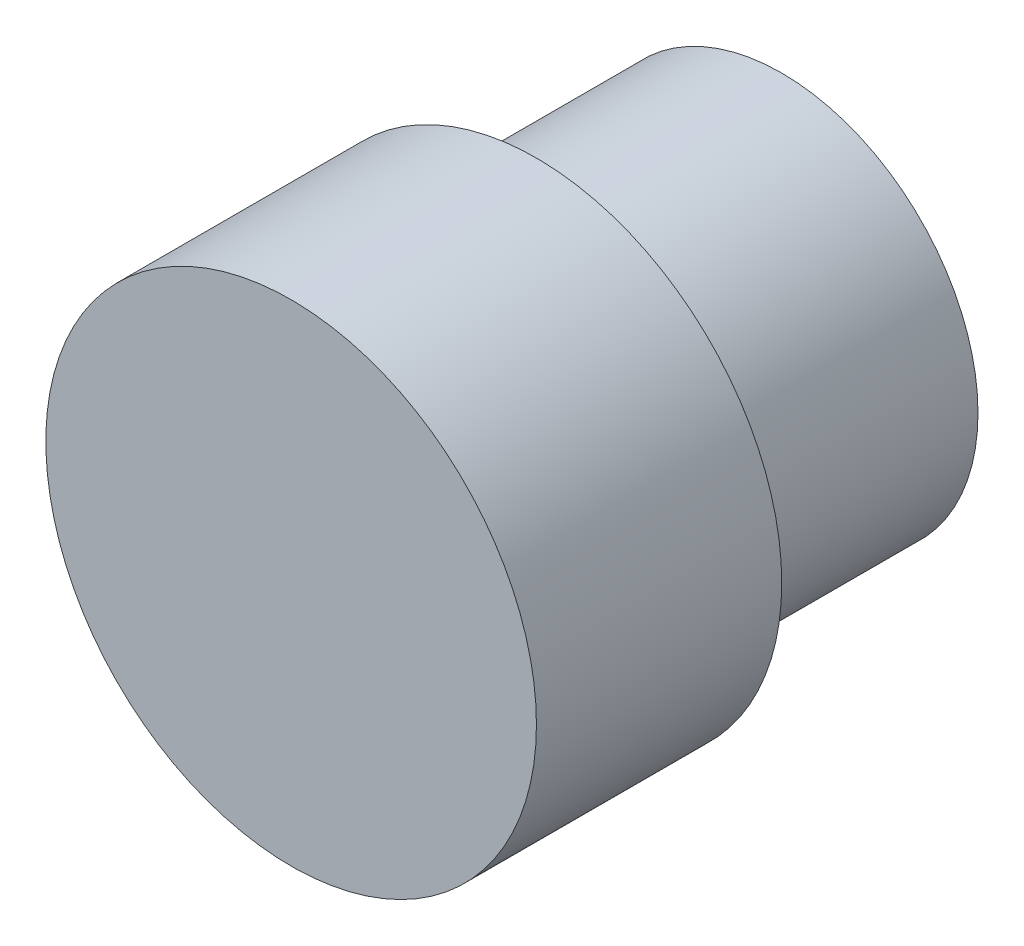
from build123d import *

# Parameters (mm, degrees)
SKETCH_1_R      = 8
EXTRUDE_1_DEPTH = 10
SKETCH_2_R      = 10
EXTRUDE_2_DEPTH = 10


with BuildPart() as part:
    # 草图1 → 凸台-拉伸1 (new body)
    with BuildSketch(Plane.XY):
        Circle(SKETCH_1_R)
    extrude(amount=-EXTRUDE_1_DEPTH)

    # 草图2 → 凸台-拉伸2 (add)
    with BuildSketch(Plane.XY):
        Circle(SKETCH_2_R)
    extrude(amount=EXTRUDE_2_DEPTH)


solid = part.part
